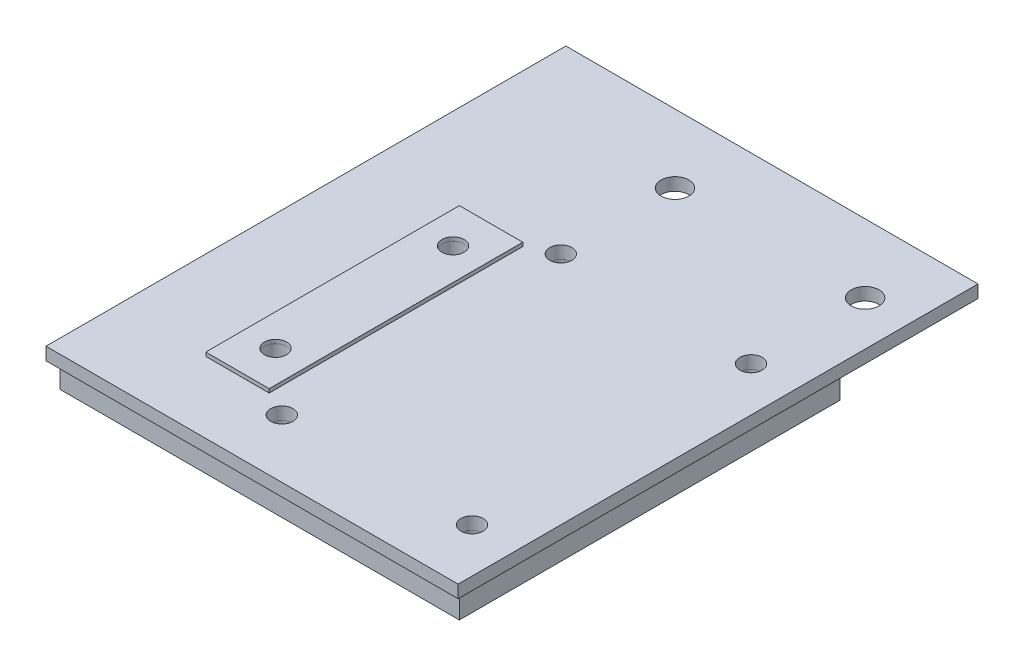
from build123d import *

# Parameters (mm, degrees)
SKETCH_1_W                   = 315
SKETCH_1_H                   = 300
EXTRUDE_1_DEPTH              = 20
SKETCH_2_W                   = 325
SKETCH_2_H                   = 410
EXTRUDE_2_DEPTH              = 10
SKETCH_3_W                   = 50
SKETCH_3_H                   = 200
EXTRUDE_3_DEPTH              = 3
SKETCH_4_W                   = 30
SKETCH_4_H                   = 100
EXTRUDE_4_DEPTH              = 30
HOLE_WIZARD_M20_1_AT_2_COUNT = 2
HOLE_WIZARD_M20_1_AT_2_PITCH = 60.207972894
HOLE_WIZARD_M20_1_AT_3_COUNT = 2
HOLE_WIZARD_M20_1_AT_3_PITCH = 185.539753153
HOLE_WIZARD_M20_1_AT_4_COUNT = 2
HOLE_WIZARD_M20_1_AT_4_PITCH = 140
HOLE_WIZARD_M20_1_AT_5_COUNT = 2
HOLE_WIZARD_M20_1_AT_5_PITCH = 265.377090194
HOLE_WIZARD_M20_1_AT_6_COUNT = 2
HOLE_WIZARD_M20_1_AT_6_PITCH = 199.060292374
SKETCH_5_R                   = 11
CUT_EXTRUDE_1_DEPTH          = 308.444710477


with BuildPart() as part:
    # 草图1 → 凸台-拉伸1 (new body)
    with BuildSketch(Plane(origin=(0, 0, 0), x_dir=(1, 0, 0), z_dir=(0, 1, 0))):
        Rectangle(SKETCH_1_W, SKETCH_1_H)
    extrude(amount=EXTRUDE_1_DEPTH)


with BuildPart() as body_2:
    # 草图2 → 凸台-拉伸2 (new body)
    with BuildSketch(Plane(origin=(0, 20, 0), x_dir=(1, 0, 0), z_dir=(0, 1, 0))):
        with Locations((0, 49)):
            Rectangle(SKETCH_2_W, SKETCH_2_H)
    extrude(amount=EXTRUDE_2_DEPTH)


with BuildPart() as body_3:
    # 草图3 → 凸台-拉伸3 (new body)
    with BuildSketch(Plane(origin=(0, 30, 0), x_dir=(1, 0, 0), z_dir=(0, 1, 0))):
        with Locations((-67.5, 0)):
            Rectangle(SKETCH_3_W, SKETCH_3_H)
    extrude(amount=EXTRUDE_3_DEPTH)


with BuildPart() as body_4:
    # 草图4 → 凸台-拉伸4 (new body)
    with BuildSketch(Plane.XZ):
        with Locations((-127.5, 0)):
            Rectangle(SKETCH_4_W, SKETCH_4_H)
    extrude(amount=EXTRUDE_4_DEPTH)


with BuildPart() as hole_wizard_m20_1_tool:
    # 草图7 → M20 螺纹孔1 (revolve)
    with BuildSketch(Plane(origin=(-67.5, 33, -70), x_dir=(0, 0, 1), z_dir=(1, 0, 0))):
        Polygon((0, 0), (0, 57.757530416), (8.75, 52.5), (8.75, 0), align=None)
    hole_wizard_m20_1 = revolve(axis=Axis((-67.5, 39.35, -70), (0, -1, 0)))


with BuildPart() as part_1:
    add(part.part)

    # M20 螺纹孔1: cut by hole_wizard_m20_1_tool
    add(hole_wizard_m20_1_tool.part, mode=Mode.SUBTRACT)


with BuildPart() as body_2_1:
    add(body_2.part)

    # M20 螺纹孔1: cut by hole_wizard_m20_1_tool
    add(hole_wizard_m20_1_tool.part, mode=Mode.SUBTRACT)


with BuildPart() as body_3_1:
    add(body_3.part)

    # M20 螺纹孔1: cut by hole_wizard_m20_1_tool
    add(hole_wizard_m20_1_tool.part, mode=Mode.SUBTRACT)


with BuildPart() as hole_wizard_m20_1_at_2_tool:
    # M20 螺纹孔1 at 2: M20 螺纹孔1 ×2
    with Locations(*[Vector(0.7474093186836596, 0, -0.6643638388299199) * (i * HOLE_WIZARD_M20_1_AT_2_PITCH) for i in range(1, HOLE_WIZARD_M20_1_AT_2_COUNT)]):
        add(hole_wizard_m20_1)


with BuildPart() as part_2:
    add(part_1.part)

    # M20 螺纹孔1 at 2: cut by hole_wizard_m20_1_at_2_tool
    add(hole_wizard_m20_1_at_2_tool.part, mode=Mode.SUBTRACT)


with BuildPart() as body_2_2:
    add(body_2_1.part)

    # M20 螺纹孔1 at 2: cut by hole_wizard_m20_1_at_2_tool
    add(hole_wizard_m20_1_at_2_tool.part, mode=Mode.SUBTRACT)


with BuildPart() as hole_wizard_m20_1_at_3_tool:
    # M20 螺纹孔1 at 3: M20 螺纹孔1 ×2
    with Locations(*[Vector(0.2425356250363329, 0, 0.970142500145332) * (i * HOLE_WIZARD_M20_1_AT_3_PITCH) for i in range(1, HOLE_WIZARD_M20_1_AT_3_COUNT)]):
        add(hole_wizard_m20_1)


with BuildPart() as part_3:
    add(part_2.part)

    # M20 螺纹孔1 at 3: cut by hole_wizard_m20_1_at_3_tool
    add(hole_wizard_m20_1_at_3_tool.part, mode=Mode.SUBTRACT)


with BuildPart() as body_2_3:
    add(body_2_2.part)

    # M20 螺纹孔1 at 3: cut by hole_wizard_m20_1_at_3_tool
    add(hole_wizard_m20_1_at_3_tool.part, mode=Mode.SUBTRACT)


with BuildPart() as hole_wizard_m20_1_at_4_tool:
    # M20 螺纹孔1 at 4: M20 螺纹孔1 ×2
    with Locations(*[(0, 0, i * HOLE_WIZARD_M20_1_AT_4_PITCH) for i in range(1, HOLE_WIZARD_M20_1_AT_4_COUNT)]):
        add(hole_wizard_m20_1)


with BuildPart() as part_4:
    add(part_3.part)

    # M20 螺纹孔1 at 4: cut by hole_wizard_m20_1_at_4_tool
    add(hole_wizard_m20_1_at_4_tool.part, mode=Mode.SUBTRACT)


with BuildPart() as body_2_4:
    add(body_2_3.part)

    # M20 螺纹孔1 at 4: cut by hole_wizard_m20_1_at_4_tool
    add(hole_wizard_m20_1_at_4_tool.part, mode=Mode.SUBTRACT)


with BuildPart() as body_3_2:
    add(body_3_1.part)

    # M20 螺纹孔1 at 4: cut by hole_wizard_m20_1_at_4_tool
    add(hole_wizard_m20_1_at_4_tool.part, mode=Mode.SUBTRACT)


with BuildPart() as hole_wizard_m20_1_at_5_tool:
    # M20 螺纹孔1 at 5: M20 螺纹孔1 ×2
    with Locations(*[Vector(0.7348034446274881, 0, 0.6782801027330657) * (i * HOLE_WIZARD_M20_1_AT_5_PITCH) for i in range(1, HOLE_WIZARD_M20_1_AT_5_COUNT)]):
        add(hole_wizard_m20_1)


with BuildPart() as part_5:
    add(part_4.part)

    # M20 螺纹孔1 at 5: cut by hole_wizard_m20_1_at_5_tool
    add(hole_wizard_m20_1_at_5_tool.part, mode=Mode.SUBTRACT)


with BuildPart() as body_2_5:
    add(body_2_4.part)

    # M20 螺纹孔1 at 5: cut by hole_wizard_m20_1_at_5_tool
    add(hole_wizard_m20_1_at_5_tool.part, mode=Mode.SUBTRACT)


with BuildPart() as hole_wizard_m20_1_at_6_tool:
    # M20 螺纹孔1 at 6: M20 螺纹孔1 ×2
    with Locations(*[Vector(0.9796027006414901, 0, -0.20094414372133138) * (i * HOLE_WIZARD_M20_1_AT_6_PITCH) for i in range(1, HOLE_WIZARD_M20_1_AT_6_COUNT)]):
        add(hole_wizard_m20_1)


with BuildPart() as part_6:
    add(part_5.part)

    # M20 螺纹孔1 at 6: cut by hole_wizard_m20_1_at_6_tool
    add(hole_wizard_m20_1_at_6_tool.part, mode=Mode.SUBTRACT)


with BuildPart() as body_2_6:
    add(body_2_5.part)

    # M20 螺纹孔1 at 6: cut by hole_wizard_m20_1_at_6_tool
    add(hole_wizard_m20_1_at_6_tool.part, mode=Mode.SUBTRACT)

    # 草图5 → 切除-拉伸1 (cut, through all)
    with BuildSketch(Plane(origin=(0, 30, 0), x_dir=(1, 0, 0), z_dir=(0, 1, 0))):
        with Locations(Location((-22.5, 200, 0), (0, 0, 270))):
            Circle(SKETCH_5_R)
        with Locations(Location((127.5, 200, 0), (0, 0, 270))):
            Circle(SKETCH_5_R)
    extrude(amount=-CUT_EXTRUDE_1_DEPTH, mode=Mode.SUBTRACT)


solid = Compound([body_4.part, body_3_2.part, part_6.part, body_2_6.part])
